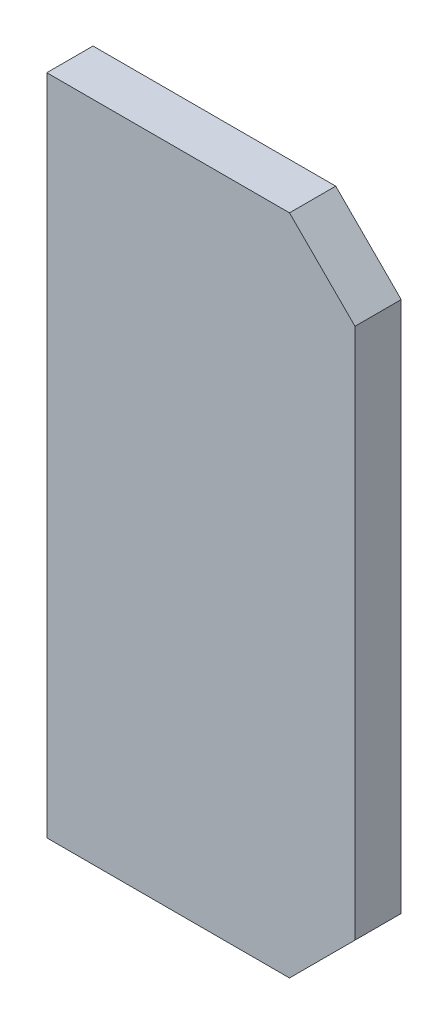
SolidWorks part; units mm, degrees
material "1023 carbon steel plate (SS)"
ref_plane "Front Plane" through (0, 0, 0) normal (0, 0, 1) x (1, 0, 0)
ref_plane "Top Plane" through (0, 0, 0) normal (0, 1, 0) x (1, 0, 0)
ref_plane "Right Plane" through (0, 0, 0) normal (1, 0, 0) x (0, 0, -1)
sketch "Sketch1" plane through (0, 0, 0) normal (0, 0, 1) x (1, 0, 0)
  line L1 (20, 43) -> (-20, 43)
  line L2 (20, 43) -> (20, -43)
  line L3 (20, -43) -> (-20, -43)
  line L4 (-20, 43) -> (-20, -43)
  line L5 (20, 43) -> (-20, -43) construction
  line L6 (20, -43) -> (-20, 43) construction
  point P0 (0, 0)
  dimension "D1" = 40
  dimension "D2" = 86
extrude "Boss-Extrude1" add sketch "Sketch1" along normal blind 6
chamfer "Chamfer1" distance 8.5 angle 45 2 edges at (20, -43, 3) (20, 43, 3)
